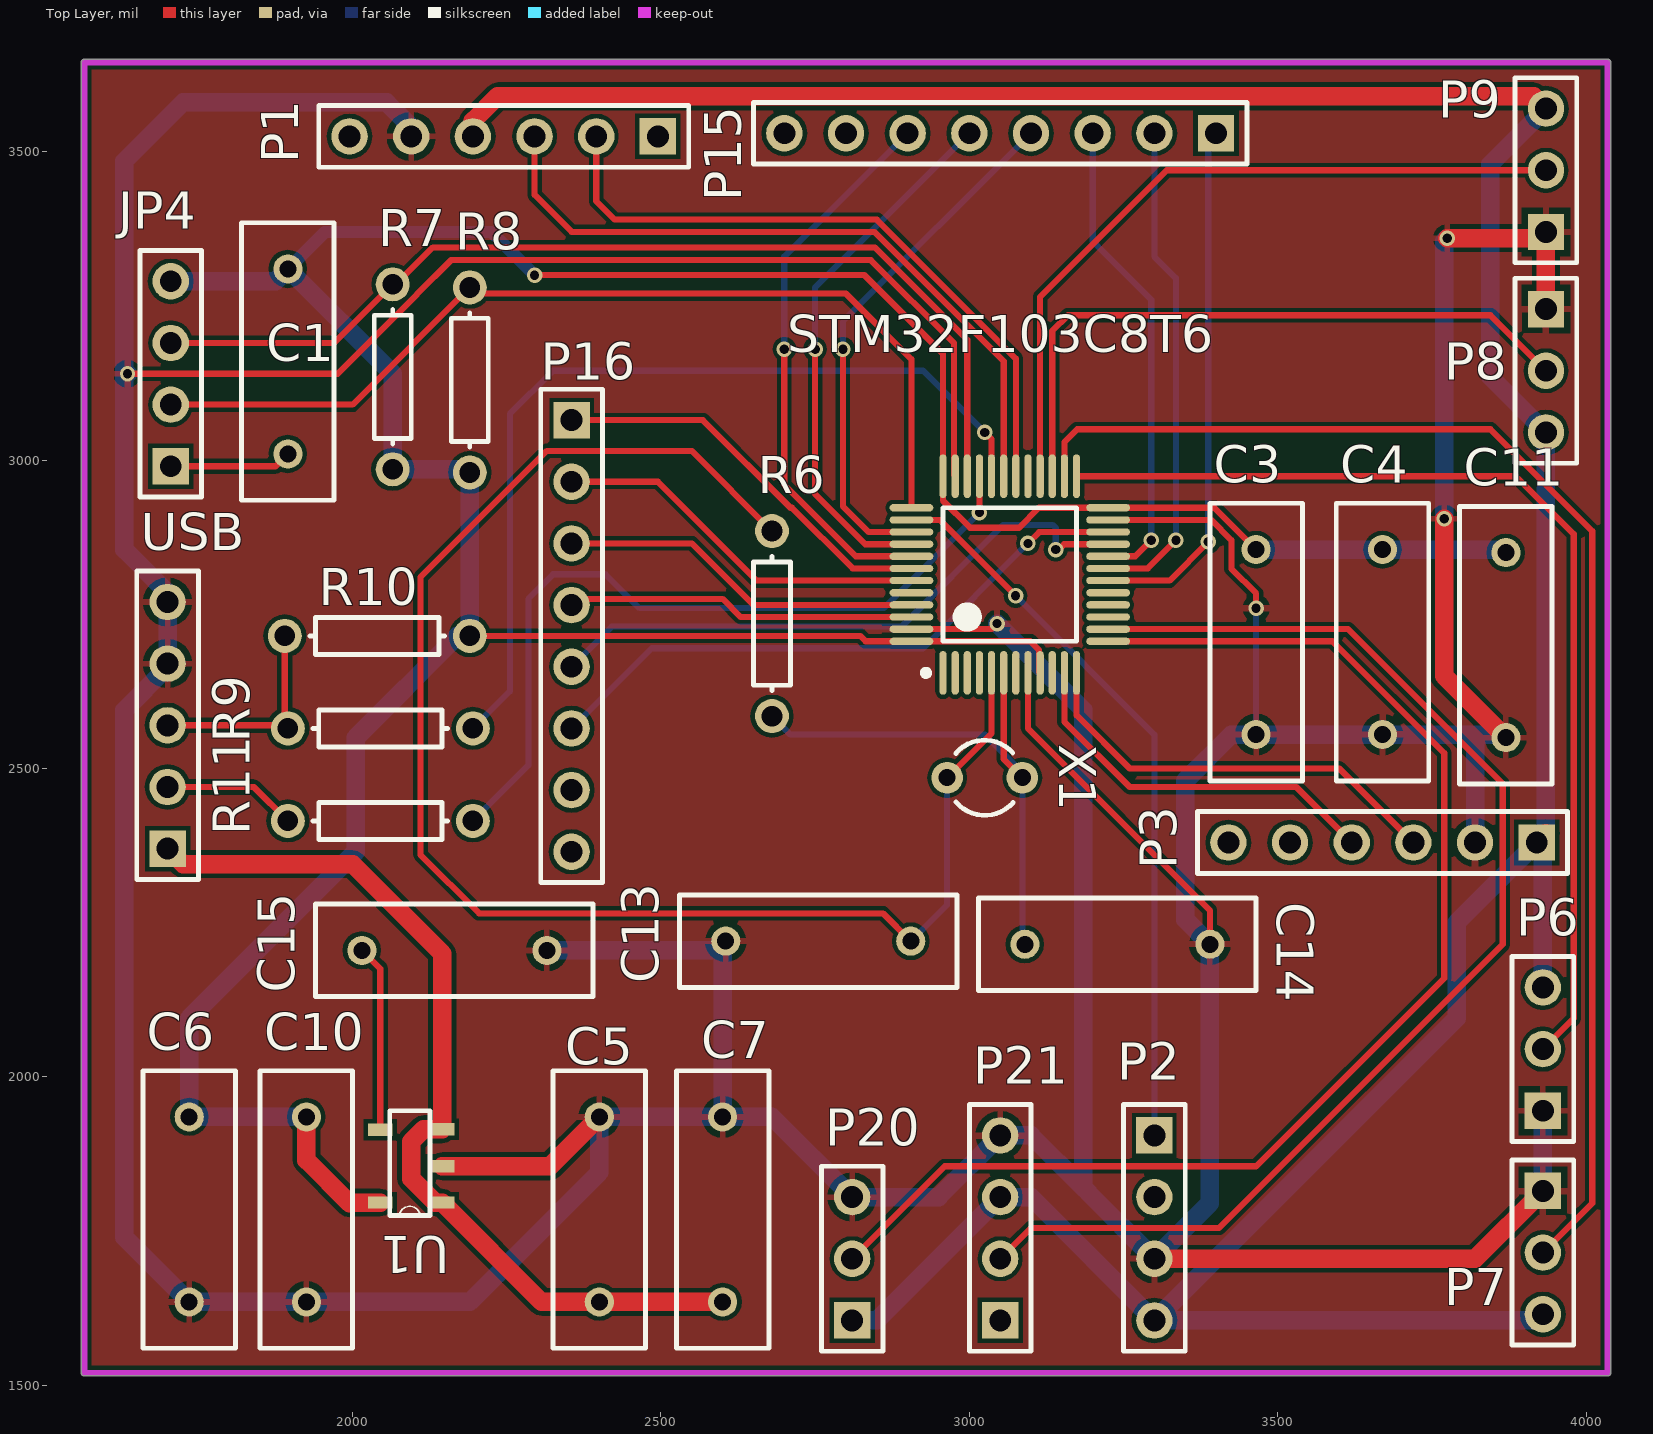
[diagram p0: Top Layer view]
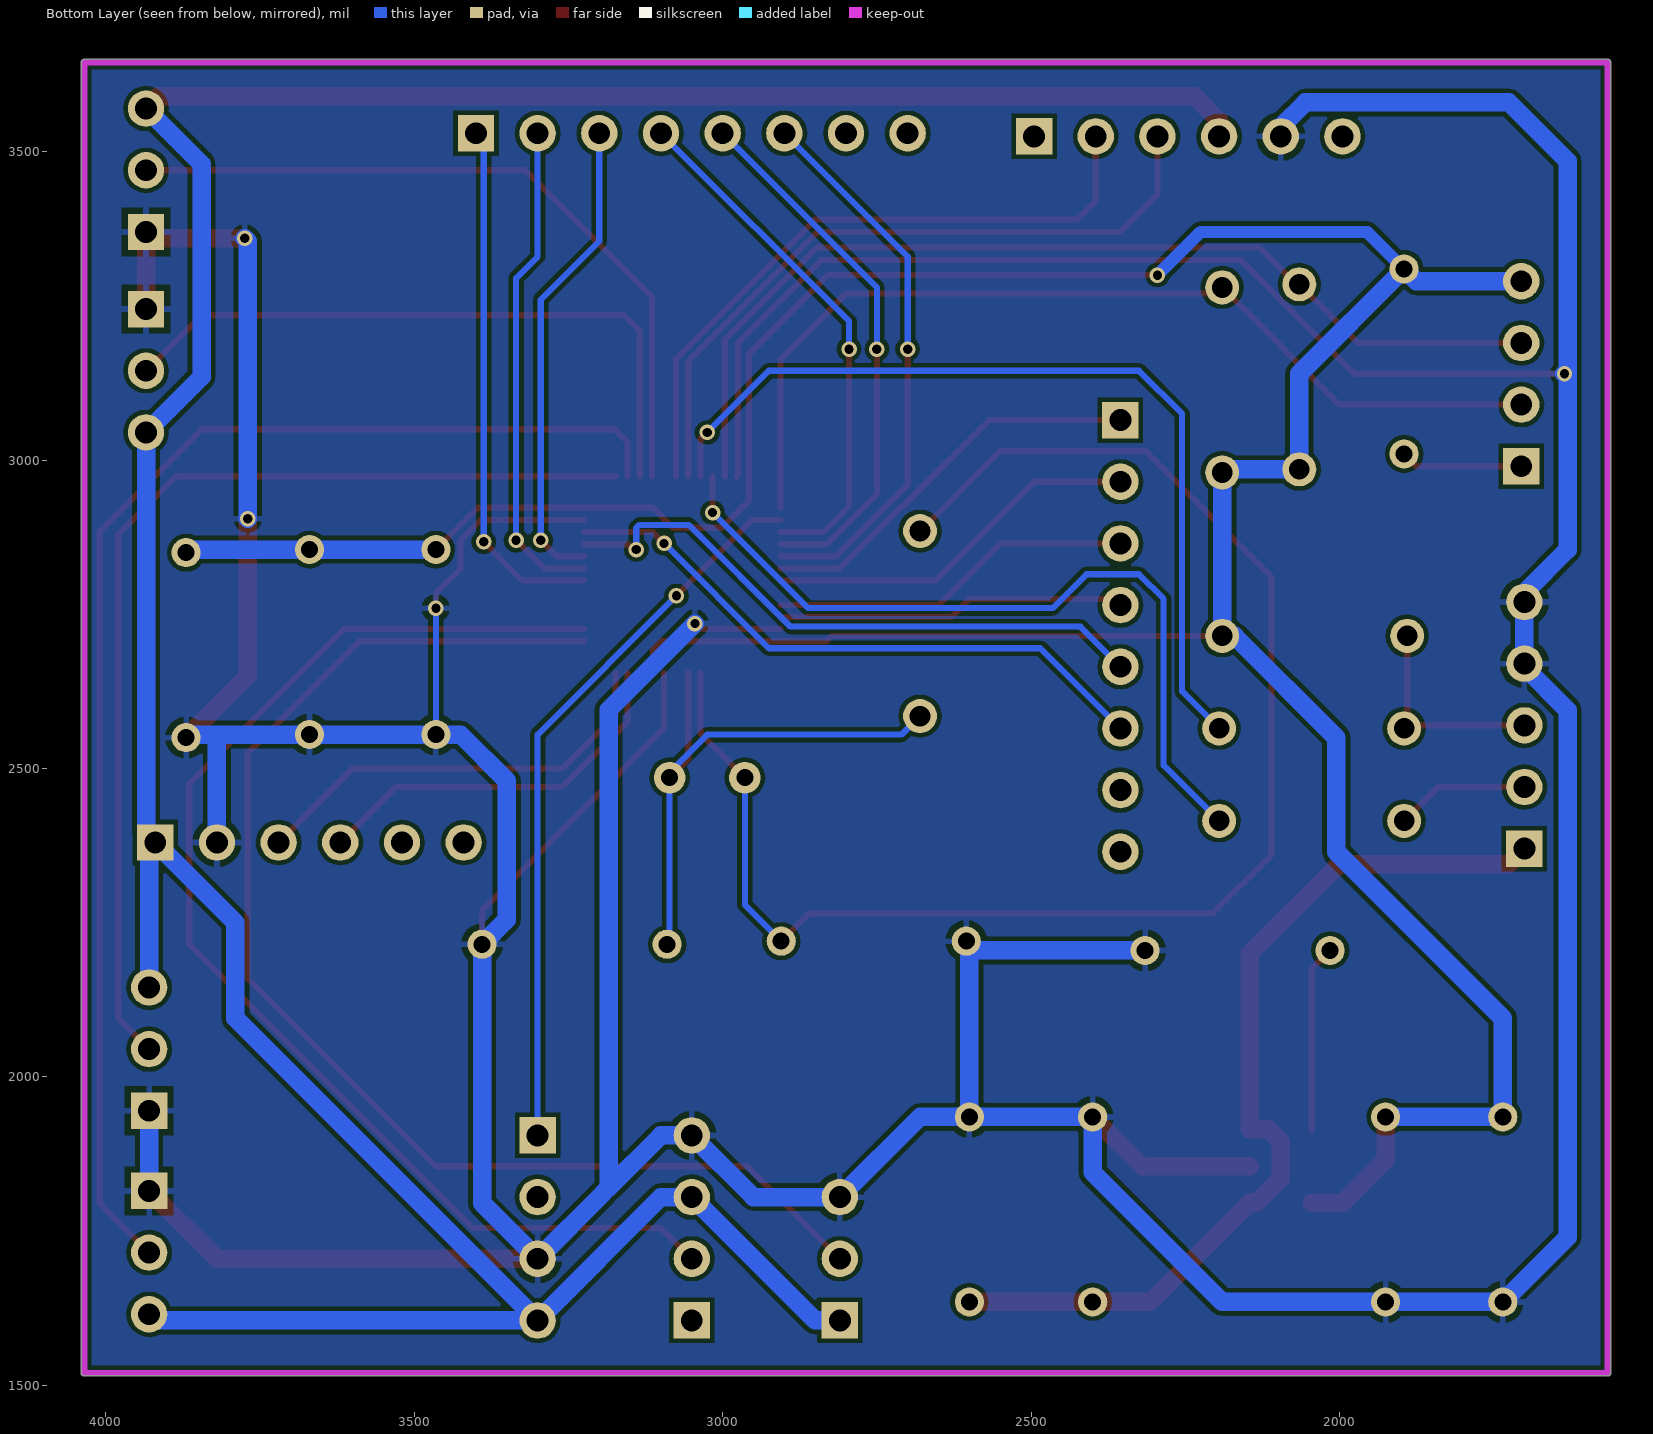
[diagram p1: Bottom Layer view, seen from below]
# Altium PCB MISC80722.PcbDoc
Units mil, origin at the board's own origin, x right, y up, seen from the top; angles counter-clockwise.
Board outline 2480.03 x 2135.03 mil, 2 copper layers (Top Layer, Bottom Layer); 33 components, 38 nets, 149 pads, 17 vias.

## Layer stack, top to bottom (the 12.6 mil dielectric is the usual default, probably not edited)
Top Solder: solder mask 0.4, Solder Resist, Dk 3.5
Top Layer: signal copper 1.4
Dielectric 1: dielectric 12.6, FR-4, Dk 4.8
Bottom Layer: signal copper 1.4
Bottom Solder: solder mask 0.4, Solder Resist, Dk 3.5

## Board outline
1559.98,1520 ccw(c1565,1520) 1565,1514.98 4035,1514.98 ccw(c4035,1520) 4040.01,1520 4040.01,3645 ccw(c4035,3645) 4035,3650.01 1565,3650.01 ccw(c1565,3645) 1559.98,3645

## Design rules (kind name [scope] priority, off if disabled: settings)
Clearance [All] p1: gap=7
PolygonConnect [All] p1: connectstyle=Relief reliefconductorwidth=10 reliefentries=4 polygonreliefangle="90 Angle" airgapwidth=10
RoutingVias [All] p1: holewidth=28 width=50 viastyle="Through Hole" minholewidth=28 minwidth=50 maxholewidth=28 maxwidth=50
SolderMaskExpansion [All] p1: expansion=4
Width [All] p1: maxlimit=50 minlimit=10 preferedwidth=20 minimp=50.000000 maximp=50.000000 favimp=50.000000
30 further rules are at their usual default settings.

## Components (designator, comment, footprint, x,y, rotation, side; value= is the part's Value field where it differs from the comment)
C1 "104" RAD-0.3 1895,3160 r90 top
C3 "Cap" RAD-0.3 3465,2705 r90 top
C4 "Cap" RAD-0.3 3670,2705 r90 top
C5 "105" RAD-0.3 2400,1785 r270 top
C6 "105" RAD-0.3 1735,1785 r90 top
C7 "104" RAD-0.3 2600,1785 r270 top
C10 "104" RAD-0.3 1925,1785 r90 top
C11 "Cap" RAD-0.3 3870,2700 r90 top
C13 "Cap" RAD-0.3 2755,2220 r180 top
C14 "Cap" RAD-0.3 3240,2215 r0 top
C15 "223" RAD-0.3 2165,2205 r180 top
JP4 "Header 4" HDR1X4 1705,2990 r90 top
P1 "Header 6" HDR1X6 2495,3525 r180 top
P2 "Header 4" HDR1X4 3300,1905 r270 top
P3 "VL53L0X" HDR1X6 3920,2380 r180 top
P6 "TTP233" HDR1X3 3930,1945 r90 top
P7 "TTP233" HDR1X3 3930,1815 r270 top
P8 "TTP233" HDR1X3 3935,3245 r270 top
P9 "TTP233" HDR1X3 3935,3370 r90 top
P15 "Header 8" HDR1X8 3400,3530 r180 top
P16 "Header 8" HDR1X8 2355,3065 r270 top
P20 "DHT11" HDR1X3 2810,1605 r90 top
P21 "OLED" HDR1X4 3050,1605 r90 top
R6 "Res1" AXIAL-0.3 2680,2735 r90 top
R7 "Res1" AXIAL-0.3 2065,3135 r90 top
R8 "Res1" AXIAL-0.3 2190,3130 r90 top
R9 "Res1" AXIAL-0.3 2045,2565 r180 top
R10 "Res1" AXIAL-0.3 2040,2715 r0 top
R11 "Res1" AXIAL-0.3 2045,2415 r180 top
STM32F103C8T6 "STM32F103C8T6" PCBComponent_1 2785.55,2894.53 r90 top
U1 "EM6211" ME6211C28M5G 2095,1860 r180 top
USB "USB-5P" HDR1X5 1700,2370 r90 top
X1 "XTAL" R38 3025,2485 r270 top

## Footprints (in the part's own frame and the unit in brackets; to place one, negate y for a bottom-side part, rotate by r counter-clockwise, add the part's x,y. Pads: shape width x height; smd on the part's side, far side on the other; paste and mask are expansions set on the pad)
AXIAL-0.3 [mm] "Axial Device, Thru-Hole; 2 Leads; 0.3 in Pin Spacing"
  round 1.4 hole 0.85: 1(-3.81,0) 2(3.81,0)
  silkscreen extent -2.77,-0.76 2.77,0.76
HDR1X3 [mm] "Connector; Header; 3 Position"
  rect 1.5x1.5 hole 0.9: 1(0,0)
  round 1.5 hole 0.9: 2(2.54,0) 3(5.08,0)
  silkscreen extent -1.27,-1.27 6.35,1.27
HDR1X4 [mm] "Connector; Header; 4 Position"
  rect 1.5x1.5 hole 0.9: 1(0,0)
  round 1.5 hole 0.9: 2(2.54,0) 3(5.08,0) 4(7.62,0)
  silkscreen extent -1.27,-1.27 8.89,1.27
HDR1X5 [mm] "Connector; Header; 5 Position"
  rect 1.5x1.5 hole 0.9: 1(0,0)
  round 1.5 hole 0.9: 2(2.54,0) 3(5.08,0) 4(7.62,0) 5(10.16,0)
  silkscreen extent -1.27,-1.27 11.43,1.27
HDR1X6 [mm] "Connector; Header; 6 Position"
  rect 1.5x1.5 hole 0.9: 1(0,0)
  round 1.5 hole 0.9: 2(2.54,0) 3(5.08,0) 4(7.62,0) 5(10.16,0) 6(12.7,0)
  silkscreen extent -1.27,-1.27 13.97,1.27
HDR1X8 [mm] "Connector; Header; 8 Position"
  rect 1.5x1.5 hole 0.9: 1(0,0)
  round 1.5 hole 0.9: 2(2.54,0) 3(5.08,0) 4(7.62,0) 5(10.16,0) 6(12.7,0) 7(15.24,0) 8(17.78,0)
  silkscreen extent -1.27,-1.27 19.05,1.27
ME6211C28M5G [mm]
  rect 1x0.5 smd paste+0 mask+0.051: 1(-1.275,1.623) 2(-1.275,0.127) 3(-1.275,-1.397) 4(1.275,-1.377) 5(1.275,1.623)
  silkscreen extent -0.77,-2.16 0.88,2.16
PCBComponent_1 [mm]
  oval 1.8x0.3 smd: 1(-6.082,-4.362) 2(-6.082,-4.862) 3(-6.082,-5.362) 4(-6.082,-5.862) 5(-6.082,-6.362) 6(-6.082,-6.862) 7(-6.082,-7.362) 8(-6.082,-7.862) 9(-6.082,-8.362) 10(-6.082,-8.862) 11(-6.082,-9.362) 12(-6.082,-9.862) 25(2.018,-9.862) 26(2.018,-9.362) 27(2.018,-8.862) 28(2.018,-8.362) 29(2.018,-7.862) 30(2.018,-7.362) 31(2.018,-6.862) 32(2.018,-6.362) 33(2.018,-5.862) 34(2.018,-5.362) 35(2.018,-4.862) 36(2.018,-4.362)
  oval 0.3x1.8 smd: 13(-4.782,-11.162) 14(-4.282,-11.162) 15(-3.782,-11.162) 16(-3.282,-11.162) 17(-2.782,-11.162) 18(-2.282,-11.162) 19(-1.782,-11.162) 20(-1.282,-11.162) 21(-0.782,-11.162) 22(-0.282,-11.162) 23(0.218,-11.162) 24(0.718,-11.162) 37(0.718,-3.062) 38(0.218,-3.062) 39(-0.282,-3.062) 40(-0.782,-3.062) 41(-1.282,-3.062) 42(-1.782,-3.062) 43(-2.282,-3.062) 44(-2.782,-3.062) 45(-3.282,-3.062) 46(-3.782,-3.062) 47(-4.282,-3.062) 48(-4.782,-3.062)
  silkscreen extent -6.21,-9.86 0.72,-3.54, body extent -5.53,-10.61 1.47,-3.61, height 1.6
R38 [mm] "Crystal, Thru-Hole; 2 Leads; Body 3.1 x 8.2 mm (Dia.xH)"
  round 1.3 hole 0.7: 1(0,1.55) 2(0,-1.55)
  silkscreen extent -1.55,-1.19 1.55,1.17
RAD-0.3 [mm] "Radial Cap, Thru-Hole; 2 Leads; 0.3 in Pin Spacing"
  round 1.2 hole 0.7: 1(-3.81,0) 2(3.81,0)
  silkscreen extent -5.71,-1.91 5.71,1.91

## Part data
C1 C5 C6 C7 C10 C15: library part Cap, "Capacitor"
C3 C4 C11 C13 C14: "Capacitor"
JP4 P2: "Header, 4-Pin"
P1: "Header, 6-Pin"
P3: library part "Header 6", "Header, 6-Pin"
P6 P7 P8 P9 P20: library part "Header 3", "Header, 3-Pin"
P15 P16: "Header, 8-Pin"
P21: library part "Header 4", "Header, 4-Pin"
R6 R7 R8 R9 R10 R11: "Resistor"
STM32F103C8T6: library part Component_1
USB: library part "Header 5", "Header, 5-Pin"
X1: "Crystal Oscillator"

## Via types
v1: diameter 25, hole 15, Top Layer to Bottom Layer, 17 vias

## Nets (pads, with @x,y where several pads share a name; then routed paths per layer and width w, separated by ;. In a path a pad name is that pad's centre, name@x,y a point inside that pad or via, vN(x,y) a via of type N, cw(c..) or ccw(c..) an arc to the next point about the centre after c; other vN are vias at no path point)
5V: C5.2 C7.2 U1.1 U1.3 USB.1 | length 1506.8
  Top Layer w30: USB.1 1725,2345 2000,2345 2145.18,2199.82 U1.3 2115,1915 2095,1895 2095,1835 2133.91,1796.09 U1.1 2306.28,1635 C5.2 C7.2
D+: R9.1 STM32F103C8T6.32 | length 1450.9
  Top Layer w10: v1(3025,3045) 3036.02,3033.98 STM32F103C8T6.32
  Bottom Layer w10: R9.1 2255,2625 2255,3075 2325,3145 2925,3145 v1(3025,3045)
D-: R11.1 STM32F103C8T6.33 | length 1291.1
  Top Layer w10: v1(3016.34,2915) STM32F103C8T6.33
  Bottom Layer w10: R11.1 2285,2505 2285,2775 2325,2815 2410,2815 2465,2760 2861.34,2760 v1(3016.34,2915)
GND: C3.1 C4.1 C5.1 C6.1 C7.1 C10.1 C11.1 C13.2 C14.2 C15.1 P1.5 P2.3 P3.2 P6.1 P7.1 P8.1 P9.1 P20.3 P21.4 STM32F103C8T6.8 STM32F103C8T6.23 STM32F103C8T6.35 STM32F103C8T6.47 U1.2 USB.4 USB.5 | length 12696.6
  Top Layer w10: v1(1635,3140) 1975.94,3140 2104.56,3268.61 2104.56,3269.56 2159.5,3324.5 2840.5,3324.5 2975.19,3189.81 2975.19,2975.76 STM32F103C8T6.35 ; STM32F103C8T6.47 3035.94,2725.94 v1(3045,2735) ; STM32F103C8T6.8 3095.08,2564.92 3390,2270 C14.2 ; STM32F103C8T6.23 3391.89,2903.11 3425,2870 3425,2824 3465,2784 v1(3465,2760)
  Top Layer w30: U1.2 2320,1855 C5.1 ; P2.3 3820,1705 P7.1 ; v1(3770,2905) 3770,2650 C11.1 ; v1(3775,3360) 3925,3360 P9.1 P8.1
  Bottom Layer w10: 3185,1820 3192.5,1812.5 ; C3.1 v1(3465,2760)
  Bottom Layer w30: v1(1635,3140) v1@1630,3145 ; P1.5 2095,3540 2055,3580 1725,3580 1630,3485 v1@1630,3145 ; C15.1 2590,2205 C13.2@2600,2215 ; C13.2 C13.2@2600,2215 ; v1(3045,2735) 3185,2595 3185,1820 3100,1905 P21.4 2950,1805 P20.3 2680,1935 C7.1 ; 3192.5,1812.5 P2.3 3390,1795 C14.2 3350,2255 3350,2480 3425,2555 C3.1 C4.1 3820,2555 ; v1(3770,2905) 3770,3355 v1(3775,3360) ; P3.2 3820,2555 ; C11.1 3865,2555 3820,2555 ; P7.1 P6.1 ; v1@1630,3145 1630,2855 1700,2785 USB.5 USB.4 1700,2664.4 1630,2594.4 1630,1740 C6.1 C10.1 2190,1635 2400,1845 C5.1 C7.1 ; C7.1 C13.2@2600,2215
KEY1: P6.2 STM32F103C8T6.25 | length 1700.8
  Top Layer w10: STM32F103C8T6.25 3886.02,2973.98 3980,2880 3980,2095 P6.2
KEY2: P7.2 STM32F103C8T6.26 | length 2191.1
  Top Layer w10: STM32F103C8T6.26 3154.13,3029.13 3175,3050 3845,3050 4010,2885 4010,1795 P7.2
KEY3: P8.2 STM32F103C8T6.27 | length 1083.9
  Top Layer w10: STM32F103C8T6.27 3134.45,3209.45 3160,3235 3845,3235 P8.2
KEY4: P9.2 STM32F103C8T6.28 | length 1196
  Top Layer w10: STM32F103C8T6.28 3114.76,3264.76 3320,3470 P9.2
NetC1_1: C1.1 JP4.1 | length 198.3
  Top Layer w10: JP4.1 1875,2990 C1.1
NetC13_1: C13.1 R6.2 STM32F103C8T6.5 X1.2 | length 2501.1
  Top Layer w10: R6.2 2550,3015 2315,3015 2110,2810 2110,2360 2205,2265 2860,2265 C13.1 ; X1.2 3036.02,2557.05 STM32F103C8T6.5
  Bottom Layer w10: C13.1 2963.98,2278.98 X1.2
NetC14_1: C14.1 R6.1 STM32F103C8T6.6 X1.1 | length 907
  Top Layer w10: STM32F103C8T6.6 3055.71,2515.31 X1.1
  Bottom Layer w10: R6.1 2710,2555 3025,2555 3086.02,2493.98 X1.1 3086.02,2218.98 C14.1
NetC15_2: C15.2 U1.4 | length 303.1
  Top Layer w10: C15.2 2044.82,2175.18 U1.4
NetR9_2: R9.2 R10.1 USB.3 | length 342.1
  Top Layer w10: USB.3 R9.2@1890,2570 ; R10.1 R9.2@1890,2570 ; R9.2 R9.2@1890,2570
NetR11_2: R11.2 USB.2 | length 217.8
  Top Layer w10: USB.2 1840,2470 R11.2
PA1: P3.4 STM32F103C8T6.11 | length 626.2
  Top Layer w10: STM32F103C8T6.11 3154.13,2575.87 3260,2470 3530,2470 P3.4
PA2: P3.3 STM32F103C8T6.12 | length 700.5
  Top Layer w10: STM32F103C8T6.12 3173.82,2586.18 3260,2500 3600,2500 P3.3
PA3: P20.2 STM32F103C8T6.13 | length 2133.5
  Top Layer w10: P20.2 2960,1855 3465,1855 3770,2160 3770,2525 3588.74,2706.26 STM32F103C8T6.13
PA4: P21.2 STM32F103C8T6.14 | length 2030.2
  Top Layer w10: P21.2 3100,1755 3405,1755 3865,2215 3865,2475 3614.06,2725.94 STM32F103C8T6.14
PA5: P21.1
PA9: P1.2 STM32F103C8T6.30 | length 1081.8
  Top Layer w10: P1.2 2395,3420 2425,3390 2850,3390 3075.39,3164.61 STM32F103C8T6.30
PA10: P1.3 STM32F103C8T6.31 | length 1153.7
  Top Layer w10: P1.3 2295,3430 2355,3370 2845.96,3370 3055.71,3160.25 STM32F103C8T6.31
PA15: P2.1 STM32F103C8T6.38 | length 1158.1
  Top Layer w10: STM32F103C8T6.38 2951.89,2903.11 v1(3075,2780)
  Bottom Layer w10: v1(3075,2780) 3300,2555 3300,1935
PB0: P15.1 STM32F103C8T6.18 | length 856.2
  Top Layer w10: STM32F103C8T6.18 3324.68,2804.68 v1(3387.5,2867.5)
  Bottom Layer w10: v1(3387.5,2867.5) 3387.5,3517.5 P15.1
PB1: P15.2 STM32F103C8T6.19 | length 803.4
  Top Layer w10: STM32F103C8T6.19 3289.37,2824.37 v1(3335,2870)
  Bottom Layer w10: P15.2 3300,3330 3335,3295 v1(3335,2870)
PB2: P15.3 STM32F103C8T6.20 | length 780.1
  Top Layer w10: STM32F103C8T6.20 3269.06,2844.06 v1(3295,2870)
  Bottom Layer w10: P15.3 3200,3355 3295,3260 v1(3295,2870)
PB3: P15.4 STM32F103C8T6.39 | length 859.7
  Top Layer w10: v1(2795,3180) 2795,2925 2836.57,2883.43 STM32F103C8T6.39
  Bottom Layer w10: v1(2795,3180) 2795,3225 P15.4
PB4: P15.5 STM32F103C8T6.40 | length 878.3
  Top Layer w10: v1(2750,3180) 2750,2945 2831.26,2863.74 STM32F103C8T6.40
  Bottom Layer w10: v1(2750,3180) 2750,3280 P15.5
PB5: P15.6 STM32F103C8T6.41 | length 907
  Top Layer w10: v1(2700,3180) 2700,2960 2815.94,2844.06 STM32F103C8T6.41
  Bottom Layer w10: v1(2700,3180) 2700,3330 P15.6
PB6: P16.1 STM32F103C8T6.42 | length 650.8
  Top Layer w10: P16.1 2567.8,3065 2710,2922.8 2712.2,2922.8 2810.63,2824.37 STM32F103C8T6.42
PB7: P16.2 STM32F103C8T6.43 | length 617.5
  Top Layer w10: P16.2 2495,2965 2655.32,2804.68 STM32F103C8T6.43
PB8: P16.3 STM32F103C8T6.45 | length 592.4
  Top Layer w10: P16.3 2550,2865 2649.69,2765.31 STM32F103C8T6.45
PB9: P16.4 STM32F103C8T6.46 | length 567.4
  Top Layer w10: P16.4 2365,2775 2600,2775 2629.37,2745.63 STM32F103C8T6.46
PB10: P16.5 STM32F103C8T6.21 | length 1006
  Top Layer w10: v1(3140,2855) 3145,2855 3153.74,2863.74 STM32F103C8T6.21
  Bottom Layer w10: P16.5 2420,2730 2890,2730 3055,2895 3135,2895 3140,2890 v1(3140,2855)
PB11: P16.6 STM32F103C8T6.22 | length 1001.9
  Top Layer w10: v1(3095,2865) 3113.43,2883.43 STM32F103C8T6.22
  Bottom Layer w10: P16.6 2485,2695 2925,2695 v1(3095,2865)
SWCLK: JP4.2 R8.2 STM32F103C8T6.37 | length 1569
  Top Layer w10: JP4.2 2000,3090 R8.2 2200,3270 2800,3270 2906.1,3163.9 STM32F103C8T6.37
SWDIO: JP4.3 R7.2 STM32F103C8T6.34 | length 1639.2
  Top Layer w10: JP4.3 1970,3190 R7.2 2070.18,3285 2130.18,3345 2846.92,3345 2996.65,3195.26 STM32F103C8T6.34
VCC: P1.4 P2.4 P3.1 P6.3 P7.3 P8.3 P9.3 P20.1 P21.3 | length 5628.5
  Top Layer w30: P1.4 2195,3550 2235,3590 3915,3590 P9.3 ; P3.1 P3.1@3935,2395
  Bottom Layer w30: P20.1 2850,1605 P21.3 3100,1805 P2.4 3920,1605 P7.3 ; P2.4@3310,1615 3790,2095 3790,2250 P3.1 ; P6.3 3930,2370 P3.1 ; P9.3 3845,3480 3845,3135 P8.3 3935,2395 P3.1
VCC3V3: C1.2 C3.2 C4.2 C6.2 C10.2 C11.2 JP4.4 R7.1 R8.1 R10.2 STM32F103C8T6.9 STM32F103C8T6.24 STM32F103C8T6.36 STM32F103C8T6.48 U1.5 | length 5727
  Top Layer w10: R10.2 2823.04,2715 2831.78,2706.26 STM32F103C8T6.48 3098.75,2706.26 3112.98,2692.02 3112.98,2656.86 STM32F103C8T6.9 ; v1(2295,3300) 2830,3300 2957.28,3172.72 STM32F103C8T6.36 2957.28,2934.37 3001.15,2890.5 3080.58,2890.5 3112.87,2922.8 STM32F103C8T6.24 3397.2,2922.8 C3.2
  Top Layer w30: C10.2 1925,1865 1995,1795 1996.09,1796.09 U1.5
  Bottom Layer w20: C1.2 1955,3370 2225,3370 v1(2295,3300)
  Bottom Layer w30: JP4.4 1875,3290 C1.2 2065,3140 R7.1 2185,2985 R8.1 R10.2 2170,2715 2005,2550 2005,2365 1735,2095 C6.2 C10.2 ; C3.2 C4.2 3865,2855 C11.2
pads on no net: P1.1 P1.6 P2.2 P3.5 P3.6 P15.7 P15.8 P16.7 P16.8 STM32F103C8T6.1 STM32F103C8T6.2 STM32F103C8T6.3 STM32F103C8T6.4 STM32F103C8T6.7 STM32F103C8T6.10 STM32F103C8T6.15 STM32F103C8T6.16 STM32F103C8T6.17 STM32F103C8T6.29 STM32F103C8T6.44

## Polygon pours and split planes (outlines as drawn)
GND on Top Layer "Top Layer-No Net" (solid, remove dead copper, pour order 4): 1380,3800 4130,3800 4230,3700 4160,3630 4160,1515 4160,1230 3900,970 3680,1190 1355,1190
GND on Bottom Layer "Top Layer-No Net" (solid, remove dead copper, pour order 6): 1365,3725 4165,3725 4165,1390 4140,1365 4110,1335 1445,1335

## Keep-outs
Keep-Out Layer:
  lines w10: 1565,1520 3995,1520 4035,1520 4035,3645 4015,3645 3995,3645 1590,3645 1565,3645 1565,1520